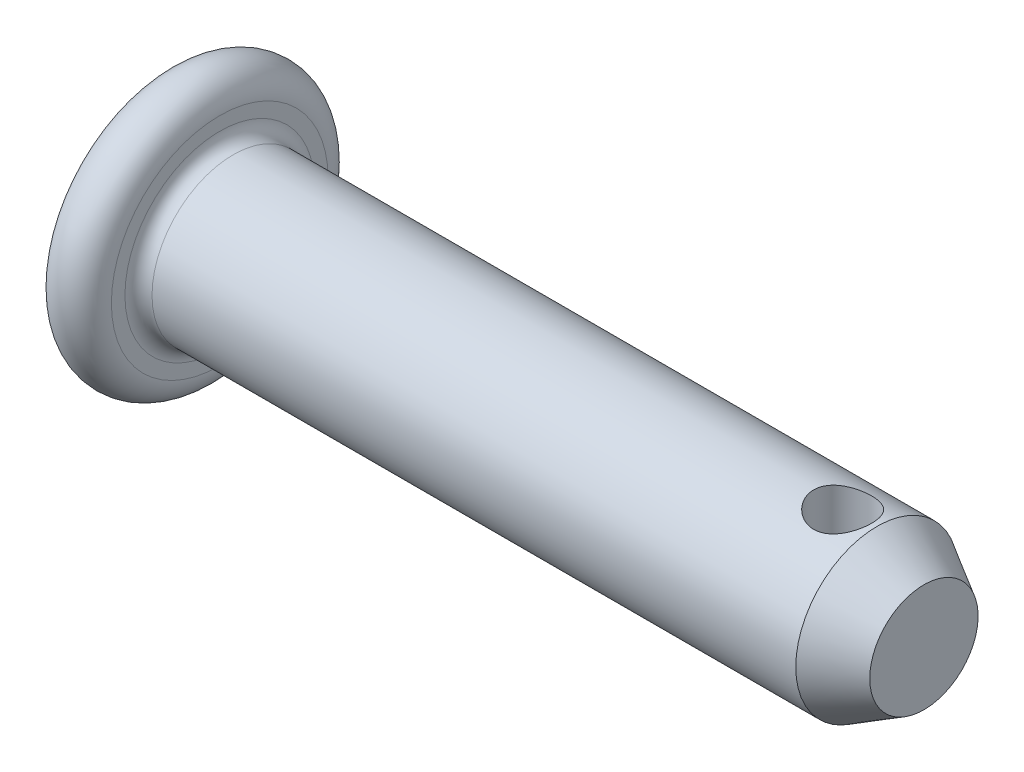
from build123d import *

# Parameters (mm, degrees)
FILLET_1_R          = 0.5
CHAMFER_1_SIZE      = 1.732050808
CHAMFER_1_SIZE2     = 1
SKETCH_2_R          = 1.07
CUT_EXTRUDE_1_DEPTH = 500


with BuildPart() as part:
    # 草图1 → Revolve 730 (revolve)
    with BuildSketch(Plane.XY, mode=Mode.PRIVATE) as revolve_730_sk:
        with BuildLine():
            Line((0, 0), (28, 0))
            Line((28, 0), (28, 3))
            Line((28, 3), (2, 3))
            Line((2, 3), (2, 4))
            ThreePointArc((2, 4), (1, 5), (0, 4))
            Line((0, 4), (0, 0))
        make_face()
    revolve(revolve_730_sk.sketch.rotate(Axis((0, 0, 0), (1, 0, 0)), 90), axis=Axis((0, 0, 0), (1, 0, 0)))

    # 圆角1
    fillet_1_edges = [part.edges().sort_by_distance(p)[0] for p in [
        (2, 0, -3),
    ]]
    fillet(fillet_1_edges, radius=FILLET_1_R)

    # 倒角1
    chamfer_1_edges = [part.edges().sort_by_distance(p)[0] for p in [
        (28, 0, -3),
    ]]
    chamfer_1_side = [part.faces().sort_by_distance(p)[0] for p in [
        (15.25, 0, -3),
    ]]
    chamfer(chamfer_1_edges, length=CHAMFER_1_SIZE, length2=CHAMFER_1_SIZE2, reference=chamfer_1_side[0])

    # 草图2 → 切除-拉伸1 (cut, symmetric)
    with BuildSketch(Plane(origin=(0, 0, 0), x_dir=(1, 0, 0), z_dir=(0, 1, 0))):
        with Locations(Location((25, 0, 0), (0, 0, 270))):
            Circle(SKETCH_2_R)
    extrude(amount=CUT_EXTRUDE_1_DEPTH, both=True, mode=Mode.SUBTRACT)


solid = part.part
